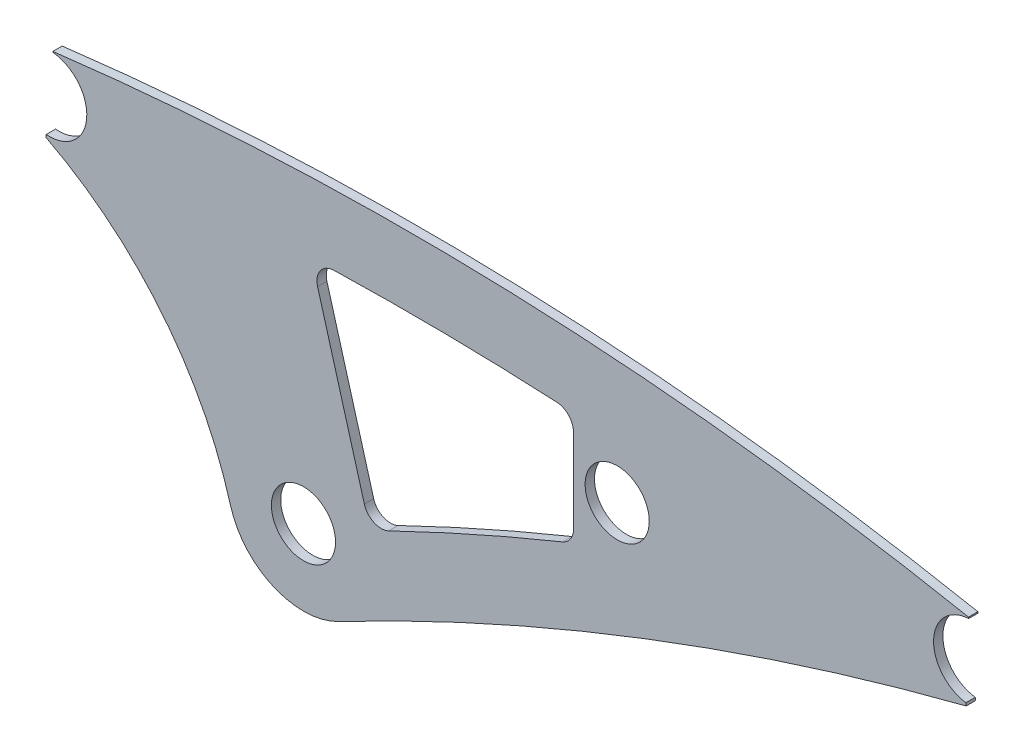
SolidWorks part; units mm, degrees
ref_plane "Front Plane" through (0, 0, 0) normal (0, 0, 1) x (1, 0, 0)
ref_plane "Top Plane" through (0, 0, 0) normal (0, 1, 0) x (1, 0, 0)
ref_plane "Right Plane" through (0, 0, 0) normal (1, 0, 0) x (0, 0, -1)
sketch "Sketch1" plane through (0, 0, 0) normal (0, 0, 1) x (1, 0, 0)
  line L0 (463, 367.628) -> (463, 222.8636)
  line L1 (104.4383, 81.2708) -> (24.2214, 364.1635)
  line L2 (-435.5, 421.2) -> (-435.5, 625.5546) construction
  line L3 (-441.4866, 352.7733) -> (-441.078, 357.4435)
  line L4 (-429.922, 484.9565) -> (-429.7949, 486.4093)
  line L5 (1144.5, 365.5) -> (1144.5, 512.5125) construction
  line L6 (1140.7088, 429.3876) -> (1140.523, 431.5116)
  line L7 (1135.9938, 302.0678) -> (1136.4, 297.4247)
  arc A0 (-125.1063, -35.3329) -> (60.2216, -115.21) centre (0, 0) ccw
  circle A1 centre (0, 0) radius 55
  arc A2 (-441.078, 357.4435) -> (-429.922, 484.9565) centre (-435.5, 421.2) ccw
  arc A3 (-125.1063, -35.3329) -> (-441.4866, 352.7733) centre (-731.3906, -206.5617) ccw
  arc A4 (1140.7088, 429.3876) -> (1135.9938, 302.0678) centre (1144.5, 365.5) ccw
  arc A5 (1140.523, 431.5116) -> (-429.7949, 486.4093) centre (182.843, -4475.9163) ccw
  arc A6 (1136.4, 297.4247) -> (60.2216, -115.21) centre (2376.4385, -4546.3656) ccw
  circle A7 centre (538, 300) radius 55
  arc A8 (444.321, 195.0817) -> (146.3672, 62.4501) centre (2376.4385, -4546.3656) ccw
  arc A9 (434.5474, 397.5881) -> (52.2809, 402.3368) centre (182.843, -4475.9163) ccw
  arc A10 (1130.8767, 419.8176) -> (4.6324, -8.8623) centre (2376.4385, -4546.3656) ccw construction
  arc A11 (104.4383, 81.2708) -> (146.3672, 62.4501) centre (133.3004, 89.4549) ccw
  arc A12 (444.321, 195.0817) -> (463, 222.8636) centre (433, 222.8636) ccw
  arc A13 (1002.7012, 334.7211) -> (-296.2206, 380.5122) centre (182.843, -4475.9163) ccw construction
  arc A14 (463, 367.628) -> (434.5474, 397.5881) centre (433, 367.628) ccw
  arc A15 (24.2214, 364.1635) -> (52.2809, 402.3368) centre (53.0835, 372.3476) cw
  arc A17 (1160.0695, 303.4227) -> (60.2216, -115.21) centre (2376.4385, -4546.3656) ccw construction
  arc A18 (1022.8617, 453.0155) -> (-308.0009, 499.9326) centre (182.843, -4475.9163) ccw construction
  dimension "D1" = 110
  dimension "D2" = 260
  dimension "D3" = 128
  dimension "D6" = 1260
  dimension "D9" = 128
  dimension "D10" = 10000
  dimension "D11" = 10000
  dimension "D14" = 110
  dimension "D18" = 30
  dimension "D4" = 421.2
  dimension "D5" = 435.5
  dimension "D7" = 365.5
  dimension "D8" = 1144.5
  dimension "D12" = 300
  dimension "D13" = 538
  dimension "D17" = 75
  dimension "D19" = 5
  dimension "D20" = 5
  dimension "D21" = 5
  dimension "D22" = 8.1
  dimension "D15" = 120
  dimension "D16" = 120
extrude "Boss-Extrude1" add sketch "Sketch1" along normal blind 16
